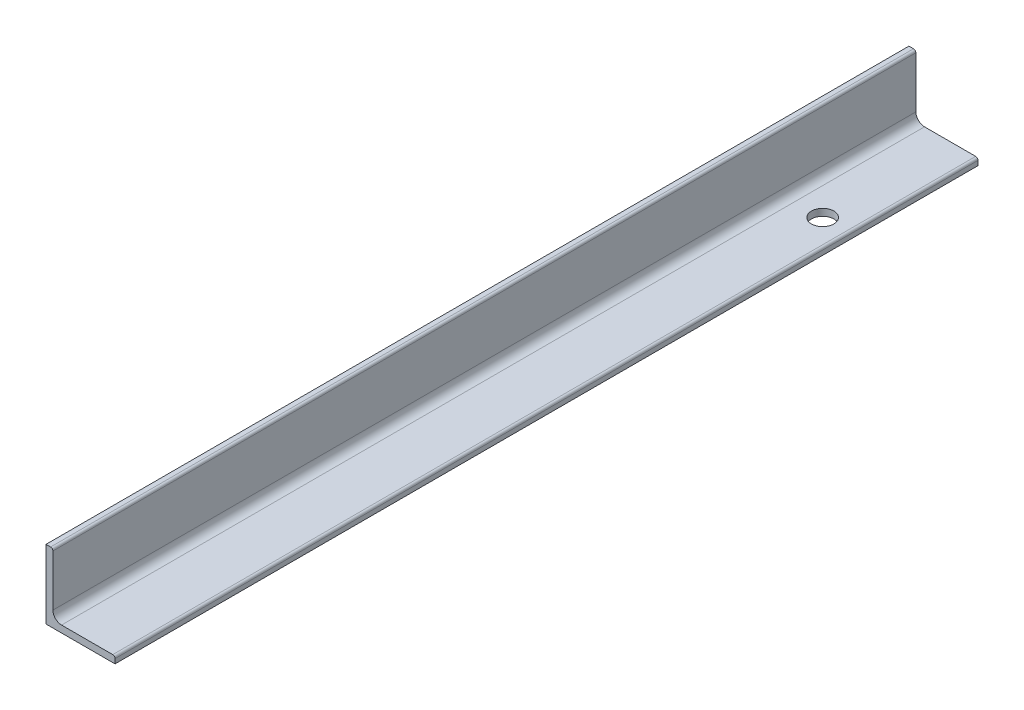
SolidWorks part; units mm, degrees
material "Q235B"
ref_plane "Plane1" through (0, 0, 0) normal (0, 0, 1) x (1, 0, 0)
ref_plane "Plane2" through (0, 0, 0) normal (0, 1, 0) x (1, 0, 0)
ref_plane "Plane3" through (0, 0, 0) normal (1, 0, 0) x (0, 0, -1)
sketch "Sketch1" plane through (0, 0, 0) normal (0, 0, 1) x (1, 0, 0)
  line L0 (0, 0) -> (0, 40)
  line L1 (0, 20) -> (4, 20) construction
  line L2 (4, 38.6667) -> (4, 9)
  line L3 (9, 4) -> (38.6667, 4)
  line L4 (20, 4) -> (20, 0) construction
  line L5 (40, 0) -> (0, 0)
  line L6 (0, 40) -> (2.6667, 40)
  line L7 (40, 0) -> (40, 2.6667)
  arc A0 (40, 2.6667) -> (38.6667, 4) centre (38.6667, 2.6667) ccw
  arc A1 (2.6667, 40) -> (4, 38.6667) centre (2.6667, 38.6667) cw
  arc A2 (9, 4) -> (4, 9) centre (9, 9) cw
  point P10 (20, 0)
  point P14 (0, 20)
  point P15 (4, 20)
  point P16 (20, 4)
  point P17 (4, 40)
  point P18 (40, 4)
  point P21 (40, 4)
  point P24 (4, 40)
extrude "Boss-Extrude1" add sketch "Sketch1" along normal blind 500 contours L3 A0 L7 L5 L0 L6 A1 L2 A2
sketch "草图1" plane through (0, 4, 0) normal (0, 1, 0) x (1, 0, 0)
  line L0 (40, -500) -> (40, 0) construction
  line L1 (9, 0) -> (38.6667, 0) construction
  line L2 (9, -500) -> (9, 0) construction
  circle A0 centre (25, -75) radius 6.5
  circle A1 centre (25, -555) radius 6.5 construction
  dimension "D1" = 13
  dimension "D2" = 15
  dimension "D3" = 75
  dimension "D5" = 480
  dimension "D4" = 16
extrude "Cut-Extrude1" cut sketch "草图1" against normal up to next
equation "\"D2@Sketch1\" = \"D1@Sketch1\" / 3"
